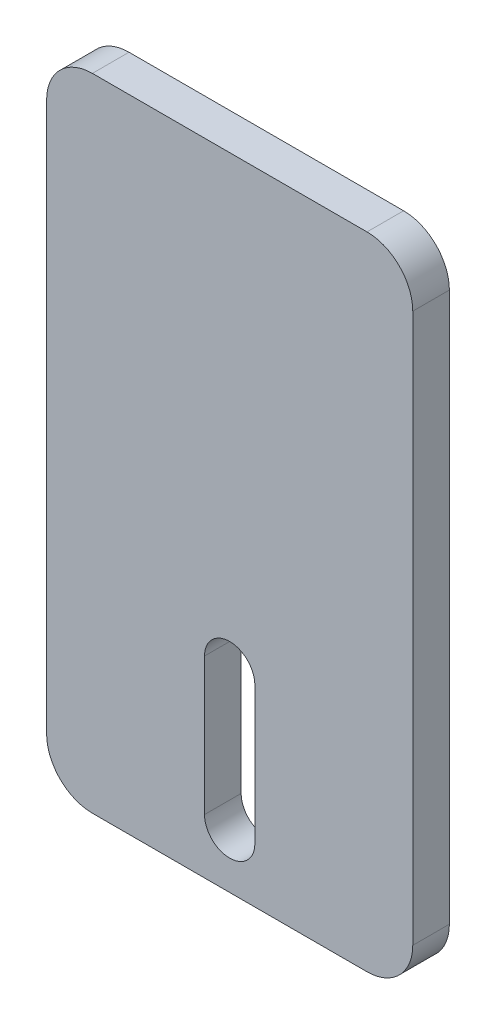
from build123d import *

# Parameters (mm, degrees)
BOSS_EXTRUDE1_DEPTH = 8
CUT_EXTRUDE1_DEPTH  = 10


with BuildPart() as part:
    # Sketch1 → Boss-Extrude1 (new body)
    with BuildSketch(Plane.XY):
        with BuildLine():
            Line((10, 0), (70, 0))
            ThreePointArc((70, 0), (77.071067812, 2.928932188), (80, 10))
            Line((80, 10), (80, 130))
            ThreePointArc((80, 130), (77.071067812, 137.071067812), (70, 140))
            Line((70, 140), (10, 140))
            ThreePointArc((10, 140), (2.928932188, 137.071067812), (0, 130))
            Line((0, 130), (0, 10))
            ThreePointArc((0, 10), (2.928932188, 2.928932188), (10, 0))
        make_face()
    extrude(amount=BOSS_EXTRUDE1_DEPTH)

    # Sketch2 → Cut-Extrude1 (cut)
    with BuildSketch(Plane.XY.offset(8)):
        with BuildLine():
            Line((34.5, 12), (34.5, 42))
            ThreePointArc((34.5, 42), (40, 47.5), (45.5, 42))
            Line((45.5, 42), (45.5, 12))
            ThreePointArc((45.5, 12), (40, 6.5), (34.5, 12))
        make_face()
    extrude(amount=-CUT_EXTRUDE1_DEPTH, mode=Mode.SUBTRACT)


solid = part.part
